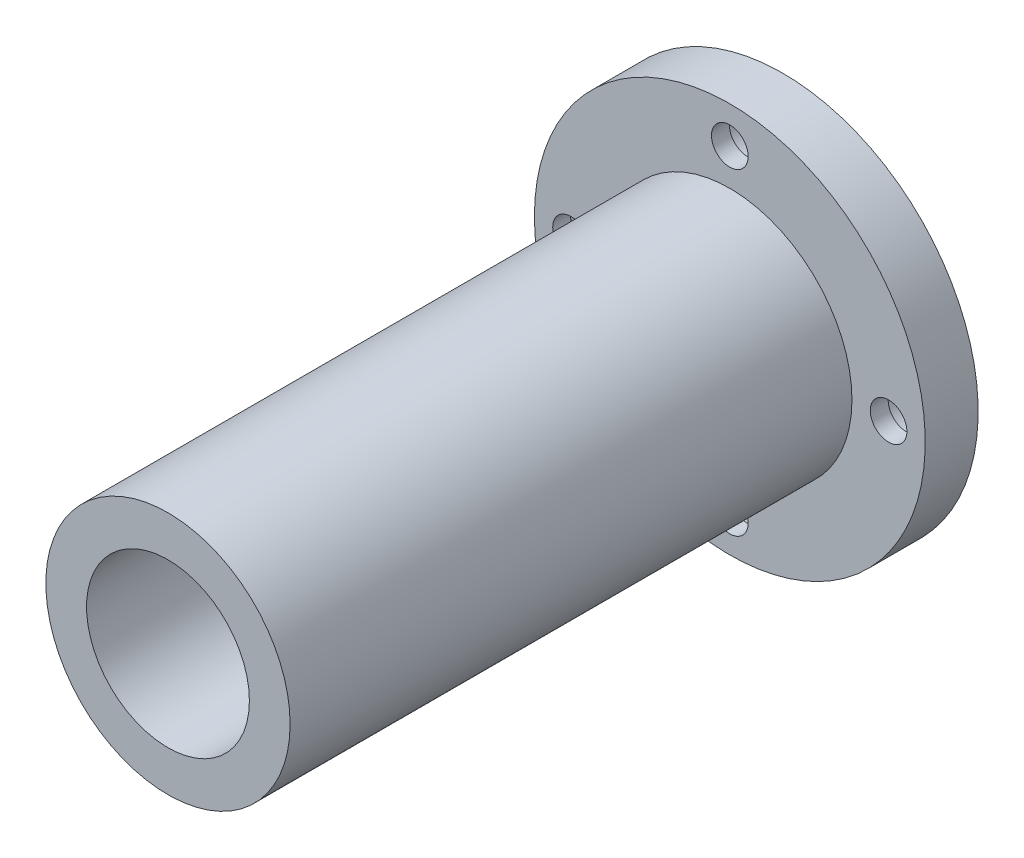
from build123d import *

# Parameters (mm, degrees)
SKETCH_1_R                   = 48
EXTRUDE_1_DEPTH              = 13
HOLE_WIZARD_M8_1_D           = 9
HOLE_WIZARD_M8_1_CBORE_D     = 14
HOLE_WIZARD_M8_1_CBORE_DEPTH = 8.6
SKETCH_3_R                   = 30
EXTRUDE_2_DEPTH              = 138
SKETCH_4_R                   = 20
CUT_EXTRUDE_3_DEPTH          = 166.556636835


with BuildPart() as part:
    # 草图1 → 拉伸1 (new body)
    with BuildSketch(Plane.XY):
        with Locations(Location((0, 0, 0), (0, 0, 180))):
            Circle(SKETCH_1_R)
    extrude(amount=EXTRUDE_1_DEPTH)

    # M8 六角凹头螺钉的柱形沉头孔1 (through all)
    with Locations(Plane(origin=(0, 39, 0), x_dir=(-1, 0, 0), z_dir=(0, 0, -1))):
        with Locations((0, 0), (-39, -39), (0, -78), (39, -39)):
            CounterBoreHole(HOLE_WIZARD_M8_1_D / 2, HOLE_WIZARD_M8_1_CBORE_D / 2, HOLE_WIZARD_M8_1_CBORE_DEPTH)

    # 草图3 → 拉伸2 (add)
    with BuildSketch(Plane.XY.offset(13)):
        Circle(SKETCH_3_R)
    extrude(amount=EXTRUDE_2_DEPTH)

    # 草图4 → 拉伸3 (cut, through all)
    with BuildSketch(Plane.XY.offset(151)):
        Circle(SKETCH_4_R)
    extrude(amount=-CUT_EXTRUDE_3_DEPTH, mode=Mode.SUBTRACT)


solid = part.part
